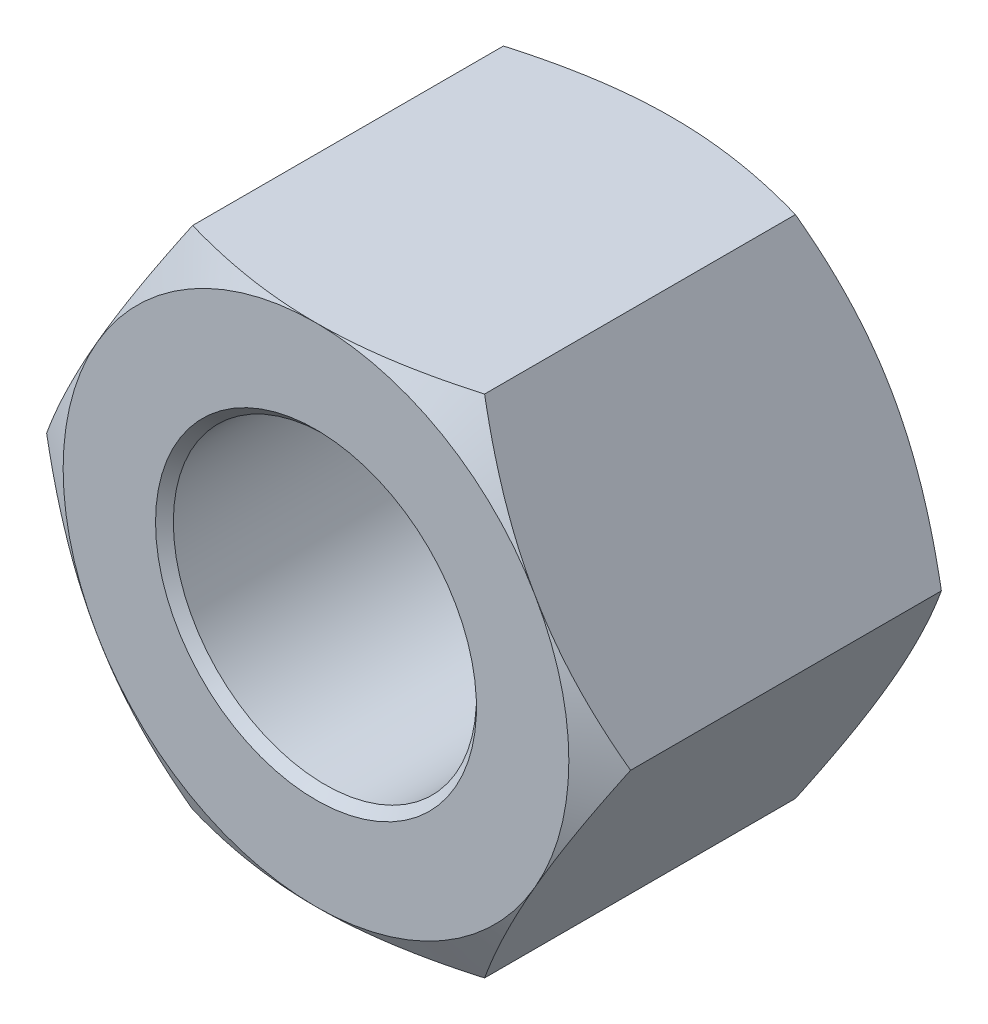
from build123d import *

# Parameters (mm, degrees)
SKETCH1_R          = 5.9175
BOSS_EXTRUDE_DEPTH = 13.9
SKETCH2_OUTSIDE_W  = 105.954
SKETCH2_OUTSIDE_H  = 102.9
SKETCH2_OUTSIDE_R  = 9.872689603
CUT_EXTRUDE1_DEPTH = 21.509509989
CUT_EXTRUDE1_DRAFT = -60
SKETCH3_OUTSIDE_W  = 105.954
SKETCH3_OUTSIDE_H  = 102.9
SKETCH3_OUTSIDE_R  = 9.872689603
CUT_EXTRUDE2_DEPTH = 21.509509989
CUT_EXTRUDE2_DRAFT = -60
CHAMFER1_SIZE      = 0.3475


with BuildPart() as part:
    # Sketch1 → Boss-Extrude (new body)
    with BuildSketch(Plane.XY):
        Polygon((5.7, 9.872689603), (-5.7, 9.872689603), (-11.4, 0), (-5.7, -9.872689603), (5.7, -9.872689603), (11.4, 0), align=None)
        Circle(SKETCH1_R, mode=Mode.SUBTRACT)
    extrude(amount=BOSS_EXTRUDE_DEPTH)


with BuildPart() as cut_extrude1_tool:
    # Sketch2 outside → Cut-Extrude1 (with draft: the straight prism first)
    with BuildSketch(Plane(origin=(0, 0, 0), x_dir=(-1, 0, 0), z_dir=(0, 0, -1))):
        Rectangle(SKETCH2_OUTSIDE_W, SKETCH2_OUTSIDE_H)
        Circle(SKETCH2_OUTSIDE_R, mode=Mode.SUBTRACT)
    extrude(amount=-CUT_EXTRUDE1_DEPTH)
    # Cut-Extrude1: the draft: its side faces are tilted about the plane it starts from
    cut_extrude1_sides = [cut_extrude1_tool.faces().sort_by_distance(p)[0] for p in [
        (0, -51.45, 10.754754995),
        (-52.977, 0, 10.754754995),
        (0, 51.45, 10.754754995),
        (52.977, 0, 10.754754995),
        (9.872689603, 0, 10.754754995),
    ]]
    draft(cut_extrude1_sides, Plane(origin=(0, 0, 0), x_dir=(-1, 0, 0), z_dir=(0, 0, -1)), CUT_EXTRUDE1_DRAFT)


with BuildPart() as part_1:
    add(part.part)

    # Cut-Extrude1: cut by cut_extrude1_tool
    add(cut_extrude1_tool.part, mode=Mode.SUBTRACT)


with BuildPart() as cut_extrude2_tool:
    # Sketch3 outside → Cut-Extrude2 (with draft: the straight prism first)
    with BuildSketch(Plane.XY.offset(13.9)):
        Rectangle(SKETCH3_OUTSIDE_W, SKETCH3_OUTSIDE_H)
        Circle(SKETCH3_OUTSIDE_R, mode=Mode.SUBTRACT)
    extrude(amount=-CUT_EXTRUDE2_DEPTH)
    # Cut-Extrude2: the draft: its side faces are tilted about the plane it starts from
    cut_extrude2_sides = [cut_extrude2_tool.faces().sort_by_distance(p)[0] for p in [
        (0, -51.45, 3.145245005),
        (52.977, 0, 3.145245005),
        (0, 51.45, 3.145245005),
        (-52.977, 0, 3.145245005),
        (-9.872689603, 0, 3.145245005),
    ]]
    draft(cut_extrude2_sides, Plane.XY.offset(13.9), CUT_EXTRUDE2_DRAFT)


with BuildPart() as part_2:
    add(part_1.part)

    # Cut-Extrude2: cut by cut_extrude2_tool
    add(cut_extrude2_tool.part, mode=Mode.SUBTRACT)

    # Chamfer1
    chamfer1_edges = [part_2.edges().sort_by_distance(p)[0] for p in [
        (-5.9175, 0, 0),
        (-5.9175, 0, 13.9),
    ]]
    chamfer(chamfer1_edges, length=CHAMFER1_SIZE)


solid = part_2.part
